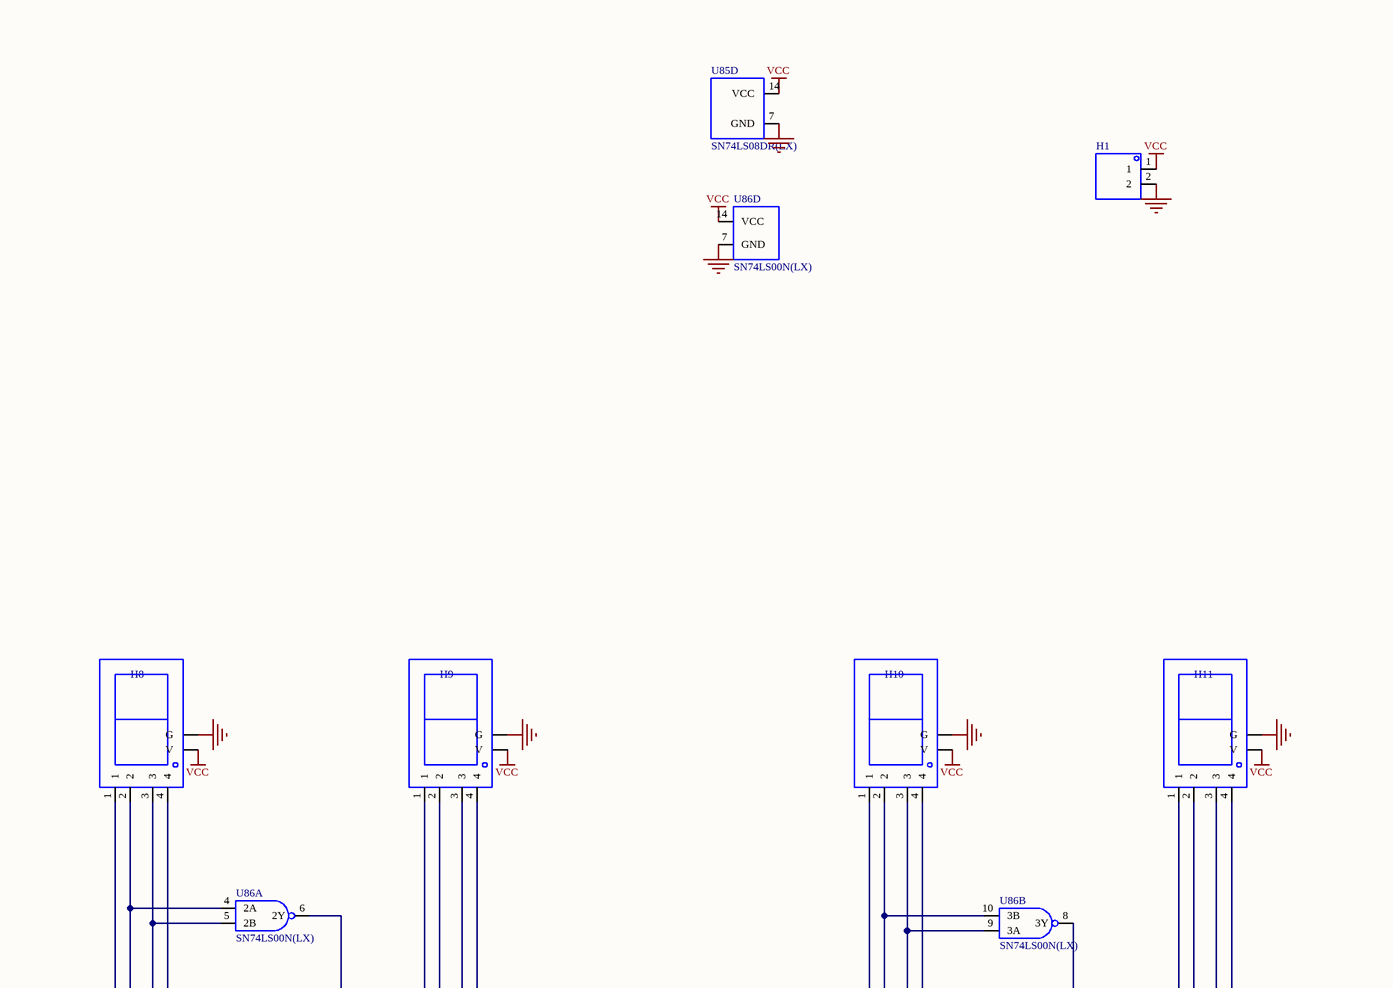
[diagram p0: MISC51760-3.schdoc, top left]
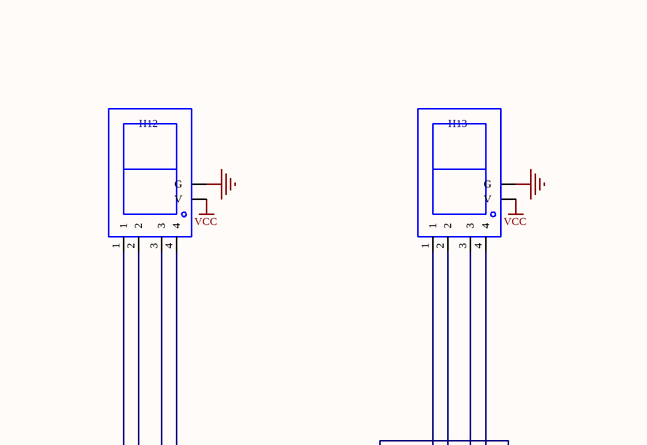
[diagram p1: MISC51760-3.schdoc, top right]
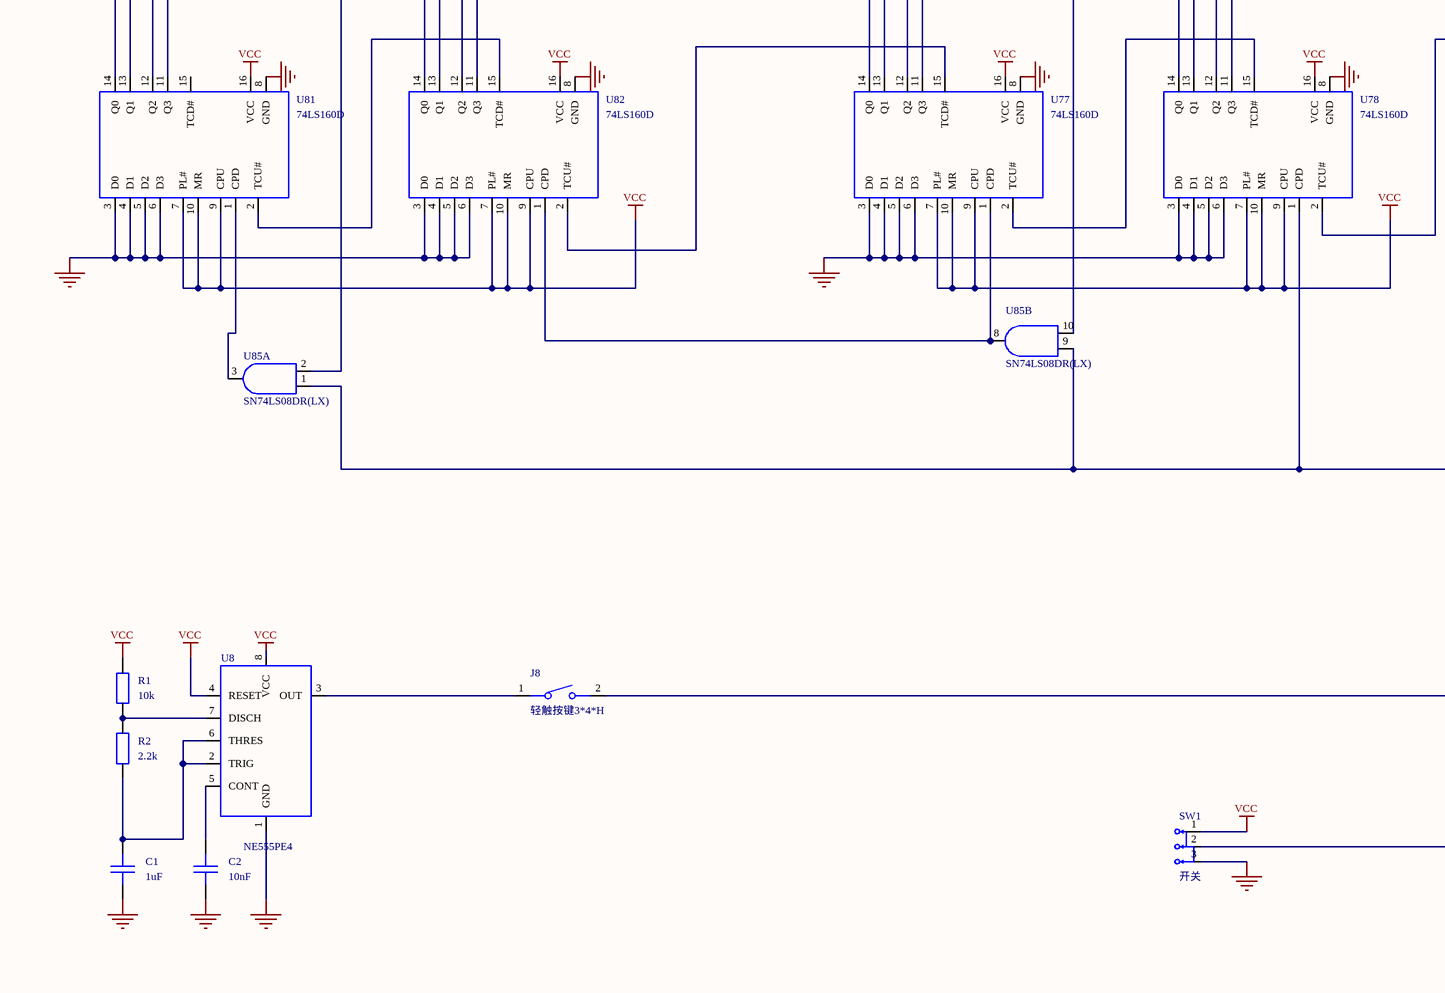
[diagram p2: MISC51760-3.schdoc, bottom left]
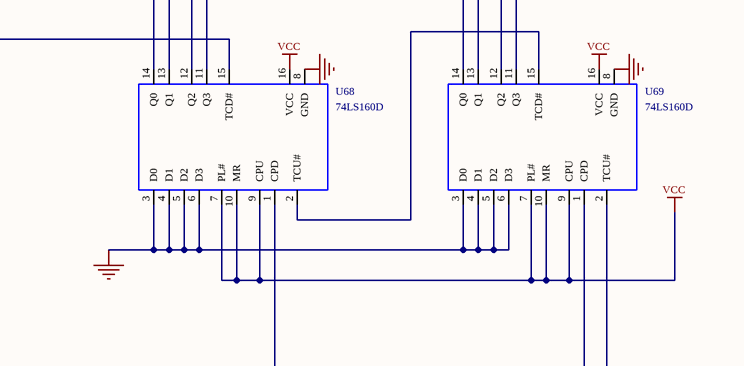
[diagram p3: MISC51760-3.schdoc, bottom right]
# Altium project MISC51760-2.PrjPcb
1 sheet, 22 parts. Net scope: global (net labels, ports and power ports of the same name join across sheets).
Board file: MISC51760.pcbdoc

## Sheet MISC51760-3.schdoc
size 178 x 98 mm; Version: V1.0; @Project Name: MISC51760; @Page Count: 1; @Update Date: 2025-06-05; @Create Date: 2025-06-05; @Schematic Name: MISC51760; @Page No: 1; @Board Name: MISC51760; @Create Time: 22:38:03; @Update Time: 20:09:27

### Parts
C1  1uF  [C0805]
C2  10nF  [C0805]
H1  (no value)  [HDR-TH_2P-P2.54-V-M-1]
H8  (no value)  [HDR-TH_6P-P2.54-V-M-1]
H9  (no value)  [HDR-TH_6P-P2.54-V-M-1]
H10  (no value)  [HDR-TH_6P-P2.54-V-M-1]
H11  (no value)  [HDR-TH_6P-P2.54-V-M-1]
H12  (no value)  [HDR-TH_6P-P2.54-V-M-1]
H13  (no value)  [HDR-TH_6P-P2.54-V-M-1]
J8  轻触按键3*4*H  [SW-SMD_L4.0-W2.9-LS5.0]
R1  10k  [R0603]
R2  2.2k  [R0603]
SW1  开关  [SW-TH_SS-12D01-GX]
U8  NE555PE4  [PDIP-8_L9.6-W6.4-P2.54-LS7.9-BL-1]
U68  74LS160D  [PDIP-16_L19.3-W6.4-P2.54-LS7.94-BL]
U69  74LS160D  [PDIP-16_L19.3-W6.4-P2.54-LS7.94-BL]
U77  74LS160D  [PDIP-16_L19.3-W6.4-P2.54-LS7.94-BL]
U78  74LS160D  [PDIP-16_L19.3-W6.4-P2.54-LS7.94-BL]
U81  74LS160D  [PDIP-16_L19.3-W6.4-P2.54-LS7.94-BL]
U82  74LS160D  [PDIP-16_L19.3-W6.4-P2.54-LS7.94-BL]
U85  SN74LS08DR(LX)  [SOIC-14_L8.7-W3.9-P1.27-LS6.0-BL]  (parts A,B,D of 4)
U86  SN74LS00N(LX)  [PDIP-14_L19.3-W6.4-P2.54-LS7.9-BL]  (parts A,B,D of 4)

### Nets
GND: C1.1 C2.1 H1.2 H8.6(G) H9.6(G) H10.6(G) H11.6(G) H12.6(G) H13.6(G) SW1.3 U8.1(GND) U68.3(D0) U68.4(D1) U68.5(D2) U68.6(D3) U68.8(GND) U69.3(D0) U69.4(D1) U69.5(D2) U69.6(D3) U69.8(GND) U77.3(D0) U77.4(D1) U77.5(D2) U77.6(D3) U77.8(GND) U78.3(D0) U78.4(D1) U78.5(D2) U78.6(D3) U78.8(GND) U81.3(D0) U81.4(D1) U81.5(D2) U81.6(D3) U81.8(GND) U82.3(D0) U82.4(D1) U82.5(D2) U82.6(D3) U82.8(GND) U85.7(GND) U86.7(GND)
VCC: H1.1 H8.5(V) H9.5(V) H10.5(V) H11.5(V) H12.5(V) H13.5(V) R1.2 SW1.1 U8.4(RESET) U8.8(VCC) U68.7(PL#) U68.9(CPU) U68.10(MR) U68.16(VCC) U69.7(PL#) U69.9(CPU) U69.10(MR) U69.16(VCC) U77.7(PL#) U77.9(CPU) U77.10(MR) U77.16(VCC) U78.7(PL#) U78.9(CPU) U78.10(MR) U78.16(VCC) U81.7(PL#) U81.9(CPU) U81.10(MR) U81.16(VCC) U82.7(PL#) U82.9(CPU) U82.10(MR) U82.16(VCC) U85.14(VCC) U86.14(VCC)
NetC1_2: C1.2 R2.1 U8.2(TRIG) U8.6(THRES)
NetC2_2: C2.2 U8.5(CONT)
NetH8_1: H8.1 U81.14(Q0)
NetH8_2: H8.2 U81.13(Q1) U86.4(2A)
NetH8_3: H8.3 U81.12(Q2) U86.5(2B)
NetH8_4: H8.4 U81.11(Q3)
NetH9_1: H9.1 U82.14(Q0)
NetH9_2: H9.2 U82.13(Q1)
NetH9_3: H9.3 U82.12(Q2)
NetH9_4: H9.4 U82.11(Q3)
NetH10_1: H10.1 U77.14(Q0)
NetH10_2: H10.2 U77.13(Q1) U86.10(3B)
NetH10_3: H10.3 U77.12(Q2) U86.9(3A)
NetH10_4: H10.4 U77.11(Q3)
NetH11_1: H11.1 U78.14(Q0)
NetH11_2: H11.2 U78.13(Q1)
NetH11_3: H11.3 U78.12(Q2)
NetH11_4: H11.4 U78.11(Q3)
NetH12_1: H12.1 U68.14(Q0)
NetH12_2: H12.2 U68.13(Q1)
NetH12_3: H12.3 U68.12(Q2)
NetH12_4: H12.4 U68.11(Q3)
NetH13_1: H13.1 U69.14(Q0)
NetH13_2: H13.2 U69.13(Q1)
NetH13_3: H13.3 U69.12(Q2)
NetH13_4: H13.4 U69.11(Q3)
NetJ8_1: J8.1 U8.3(OUT)
NetJ8_2: J8.2 U69.1(CPD)
NetR1_1: R1.1 R2.2 U8.7(DISCH)
NetSW1_2: SW1.2 U68.1(CPD) U69.2(TCU#) U78.1(CPD) U85.1(1A) U85.9(3A)
NetU68_2: U68.2(TCU#) U69.15(TCD#)
NetU68_15: U68.15(TCD#) U78.2(TCU#)
NetU77_1: U77.1(CPD) U82.1(CPD) U85.8(3Y)
NetU77_2: U77.2(TCU#) U78.15(TCD#)
NetU77_15: U77.15(TCD#) U82.2(TCU#)
NetU81_1: U81.1(CPD) U85.3(1Y)
NetU81_2: U81.2(TCU#) U82.15(TCD#)
NetU85_2: U85.2(1B) U86.6(2Y)
NetU85_10: U85.10(3B) U86.8(3Y)

Not connected (* = marked no-connect by the designer): U81 15(TCD#)

### Notes on the sheet
- 2025-06-05
- 原理图
- P1
- 版本
- 尺寸
- 页
- 共
- A4
- 1

### Library data of the parts
C1 C2 = CAP_0805: ConvertToPcb: yes; SymbolName: CapAcitance; ModelId: 1ba041120af144c991958decab20d241; ModelName: C0805_L2.0-W1.3-H1.3; ModelTransform: 78.74,51.181,0,0,0,0,0,0.0005,0; Device: CAP_0805; AddInBom: yes; Supplier Footprint: 0805; FootprintName: C0805
  C1: Value: 1uF
  C2: Value: 10nF
H1 = HDR-M_2.54_1x2P: Symbol: 210S-1*2P L=11.6MMGold-plated black; ConvertToPcb: yes; ModelId: 79b2e9f2d70a4d68a1b7098f27c6d4c5; ModelName: HDR-M-2.54_1x2; ModelTransform: 200,100,0,0,0,0,0,0,-118.11; Device: HDR-M_2.54_1x2P; AddInBom: yes; SupplierPart: C124375; Supplier Footprint: 插件; FootprintName: HDR-TH_2P-P2.54-V-M-1
H8-H13 = HDR-M_2.54_1x6P: Symbol: Header-Male-2.54_1x6; ConvertToPcb: yes; ModelId: 60739dffc9b04830a286435b0fefbd4a; ModelName: HDR2.54-M-LI-1X6P; ModelTransform: 599.999,100,0,0,0,0,0,0,-118.11; Device: HDR-M_2.54_1x6P; AddInBom: yes; SupplierPart: C37208; Supplier Footprint: 插件; FootprintName: HDR-TH_6P-P2.54-V-M-1
J8 = 轻触按键3*4*H: AddInBom: yes; ModelId: 63599cce708d48afbce1b0db00354477; ModelName: SW-SMD_L4.0-W2.9-H2-LS5.0; ModelTransform: 196.85,114.173,0,0,0,0,0,0,0; Symbol: 轻触按键3*4*H; Device: 轻触按键3*4*H; LCSC Part Name: 轻触按键3*4*H; SupplierPart: C9900017573; ManufacturerPart: 轻触按键3*4*H; Supplier Footprint: 轻触按键3*4*2.5; Supplier: LCSC; ConvertToPcb: yes; FootprintName: SW-SMD_L4.0-W2.9-LS5.0
R1 R2 = Res_0603: Symbol: 电阻; ConvertToPcb: yes; ModelId: fc143cca1e79419f9cd78b61e9279f08; ModelTransform: 31.8897,63.7794,0,90,0,0,0,0,0; Device: Res_0603; AddInBom: yes; Supplier Footprint: 0603; FootprintName: R0603; ModelName: R0603
  R1: Value: 10k
  R2: Value: 2.2k
SW1 = 开关: AddInBom: yes; ModelId: 46ec4e06866345239622c383c14b792d; ModelTransform: 346.456,153.543,0,0,0,0,-0.005,0,-169.291; Symbol: 开关; Device: 开关; LCSC Part Name: 开关; SupplierPart: C9900023015; ManufacturerPart: 开关; Supplier Footprint: SW-TH; Supplier: LCSC; ConvertToPcb: yes; FootprintName: SW-TH_SS-12D01-GX; ModelName: SW-TH_SS-12D01-GX
U8 = NE555PE4: 单精度计时器 8-PDIP 0 to 70; Manufacturer: TI(德州仪器); AddInBom: yes; ModelId: 1b8eaf096e7944deafe216467068c10e; ModelTransform: 377.952,318.897,0,0,0,0,0,0,-118.11; Symbol: NE555PE4; Device: NE555PE4; LCSC Part Name: NE555PE4; SupplierPart: C2859604; ManufacturerPart: NE555PE4; Supplier Footprint: PDIP-8; Datasheet: https://www.ti.com/cn/lit/gpn/sa555; Supplier: LCSC; ConvertToPcb: yes; FootprintName: PDIP-8_L9.6-W6.4-P2.54-LS7.9-BL-1; ModelName: PDIP-8_L9.6-W6.4-P2.54-LS7.9-BL-1
U68 U69 U77 U78 U81 U82 = SN74LS192N(LX): 工作电压:2V~6V;元件数:1;触发沿:上升沿;计数速率:24MHz;; Manufacturer: LX(灵星芯微); AddInBom: yes; Logic Type: 十进制计数器; Direction: 向下计数器;向上计数器; Supply Voltage: 2V~6V; Number of Elements: 1; Trigger Type: 上升沿; Reset Style: 异步; Timing mode: 同步; Count Rate: 24MHz; ModelId: 96ff5d01b3074dd183bcbc4cd00a63de; ModelTransform: 759.841,322.44,0,0,0,0,0,0,-137.795; Manufacturer Part: 74LS160D; Symbol: SN74LS192N(LX); Device: SN74LS192N(LX); LCSC Part Name: SN74LS192N(LX); SupplierPart: C22449628; Supplier Footprint: DIP-16; JLCPCB Part Class: 扩展库; Datasheet: https://atta.szlcsc.com/upload/public/pdf/source/20240603/08E986A67799FBEA7E290B817BAE27A9.pdf; Supplier: LCSC; ConvertToPcb: yes; Operating Temperature: -40℃~+85℃; FootprintName: PDIP-16_L19.3-W6.4-P2.54-LS7.94-BL; ModelName: PDIP-16_L19.3-W6.4-P2.54-LS7.94-BL
U85 = SN74LS08DR(LX): 逻辑类型:与门;通道数:4;电源电压:2V~6V;静态电流(最大值):2uA;最大传播延迟:15ns@6V;; Manufacturer: LX(灵星芯微); Relevance: []; AddInBom: yes; Logic Gate Type: 与门; Number of Channels: 4; Supply Voltage: 2V~6V; Quiescent Current (Max): 2uA; Sink Current: 5.2mA; High Level Range (VIH): 1.5V~4.2V; Low Level Range (VIL): 500mV~1.8V; ModelId: 8dbf5b715d42428c85558507ae5a252b; ModelName: SOIC-14_L8.6-W3.9-H1.8-LS6.0-P1.27; ModelTransform: 338.583,236.22,0,0,0,0,0,-0.001,0; Device: SN74LS08DR(LX); LCSC Part Name: 集成电路; SupplierPart: C22384802; ManufacturerPart: SN74LS08DR(LX); Supplier Footprint: SOP-14; Datasheet: https://atta.szlcsc.com/upload/public/pdf/source/20240417/39D5CB7746FCA2B194C58FD97B1F3E32.pdf; Supplier: LCSC; ConvertToPcb: yes; Source Current: 5.2mA; Series: 74LS系列; Propagation Delay Time: 15ns@6V; Operating Temperature: -40℃~+125℃; SymbolName: SN74LS08DR(LX); FootprintName: SOIC-14_L8.7-W3.9-P1.27-LS6.0-BL
U86 = SN74LS00N(LX): 逻辑类型:与非门;通道数:4;电源电压:2V~6V;静态电流(最大值):2uA;最大传播延迟:7ns@6V;; Manufacturer: LX(灵星芯微); Relevance: []; AddInBom: yes; Logic Gate Type: 与非门; Number of Channels: 4; Supply Voltage: 2V~6V; Quiescent Current (Max): 2uA; Sink Current: 5.2mA; High Level Range (VIH): 1.2V~3.2V; Low Level Range (VIL): 800mV~2.8V; Propagation Delay Time: 7ns@6V; ModelId: ed65e85d32ac41798f005e95ecc59a64; ModelTransform: 759.841,309.842,0,0,0,0,0,0,-118.11; Device: SN74LS00N(LX); LCSC Part Name: SN74LS00N(LX); SupplierPart: C22374089; ManufacturerPart: SN74LS00N(LX); Supplier Footprint: DIP-14; JLCPCB Part Class: 扩展库; Datasheet: https://atta.szlcsc.com/upload/public/pdf/source/20240402/5C5C61F6856D913ABEF0173ADDE42D20.pdf; Supplier: LCSC; ConvertToPcb: yes; Source Current: 5.2mA; Series: 74LS系列; Operating Temperature: -40℃~+125℃; SymbolName: SN74LS00N(LX); FootprintName: PDIP-14_L19.3-W6.4-P2.54-LS7.9-BL; ModelName: PDIP-14_L19.3-W6.4-P2.54-LS7.9-BL